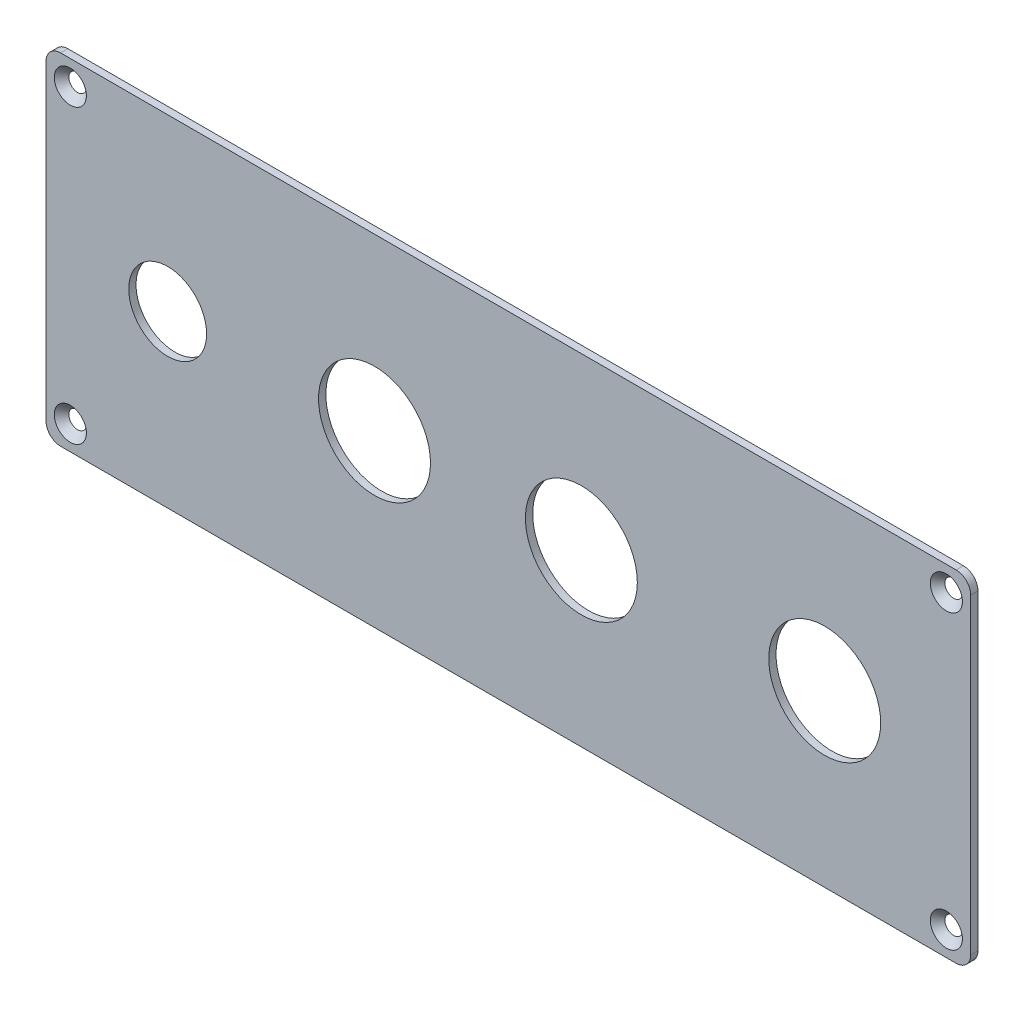
SolidWorks part; units mm, degrees
material "Q235"
ref_plane "前视基准面" through (0, 0, 0) normal (0, 0, 1) x (1, 0, 0)
ref_plane "上视基准面" through (0, 0, 0) normal (0, 1, 0) x (1, 0, 0)
ref_plane "右视基准面" through (0, 0, 0) normal (1, 0, 0) x (0, 0, -1)
sketch "草图1" plane through (0, 0, 0) normal (0, 0, 1) x (1, 0, 0)
  line L1 (-95, 35) -> (95, 35)
  line L2 (-95, 35) -> (-95, -35)
  line L3 (-95, -35) -> (95, -35)
  line L4 (95, 35) -> (95, -35)
  line L5 (-95, 35) -> (95, -35) construction
  line L6 (-95, -35) -> (95, 35) construction
  point P0 (0, 0)
  dimension "D1" = 190
  dimension "D2" = 70
extrude "凸台-拉伸1" add sketch "草图1" along normal blind 1.5
fillet "圆角1" radius 3 4 edges at (-95, 35, 0.75) (-95, -35, 0.75) (95, -35, 0.75) (95, 35, 0.75)
sketch "草图2" plane through (0, 0, 1.5) normal (0, 0, 1) x (1, 0, 0)
  line L0 (-95, 0) -> (95, 0) construction
  line L1 (-95, 32) -> (-95, -32) construction
  line L2 (95, -32) -> (95, 32) construction
  circle A0 centre (15, 0) radius 11.5
  circle A1 centre (-27.5, 0) radius 11.5
  circle A2 centre (65, 0) radius 11.5
  circle A3 centre (-70, 0) radius 8
  dimension "D1" = 30
  dimension "D2" = 50
  dimension "D3" = 23
  dimension "D4" = 23
  dimension "D5" = 42.5
  dimension "D6" = 23
  dimension "D7" = 16
  dimension "D8" = 42.5
extrude "切除-拉伸1" cut sketch "草图2" against normal blind 1.5
sketch "草图3" plane through (0, 0, 1.5) normal (0, 0, 1) x (1, 0, 0)
  line L0 (0, 35) -> (0, -35) construction
  line L1 (92, 35) -> (-92, 35) construction
  line L2 (-92, -35) -> (92, -35) construction
  line L3 (95, -32) -> (95, 32) construction
  line L4 (-90, -30) -> (90, -30)
  line L5 (-90, -30) -> (-90, 30)
  line L6 (-90, 30) -> (90, 30)
  line L7 (90, -30) -> (90, 30)
  line L8 (-90, -30) -> (90, 30) construction
  line L9 (-90, 30) -> (90, -30) construction
  point P6 (0, 0)
  dimension "D1" = 5
  dimension "D2" = 5
hole_wizard "打孔尺寸根据十字槽半沉头木螺钉的类型1" positions "草图5" profile "草图4" countersink size "M3" standard "GB" end condition through all
sketch "草图5" plane through (0, 0, 1.5) normal (0, 0, 1) x (1, 0, 0)
  point P1 (-90, 30)
  point P4 (-90, -30)
  point P7 (90, -30)
  point P10 (90, 30)
sketch "草图4" plane through (-90, 30, 1.5) normal (1, 0, 0) x (0, -1, 0)
  line L0 (0, 0) -> (0, 1.5)
  line L1 (0, 1.5) -> (1.7, 1.5)
  line L2 (1.7, 1.5) -> (1.7, 1.6)
  line L3 (1.7, 1.6) -> (3.3, 0)
  line L5 (3.3, 0) -> (0, 0)
  line L6 (-1.7, 1.6) -> (-3.3, 0) construction
  line L11 (0, -6.35) -> (0, 107.95) construction
  dimension "通孔孔直径" = 3.4
  dimension "通孔孔深度" = 1.5
  dimension "近端锥形沉头孔直径" = 6.6
  dimension "近端锥形沉头孔角度" = 90
